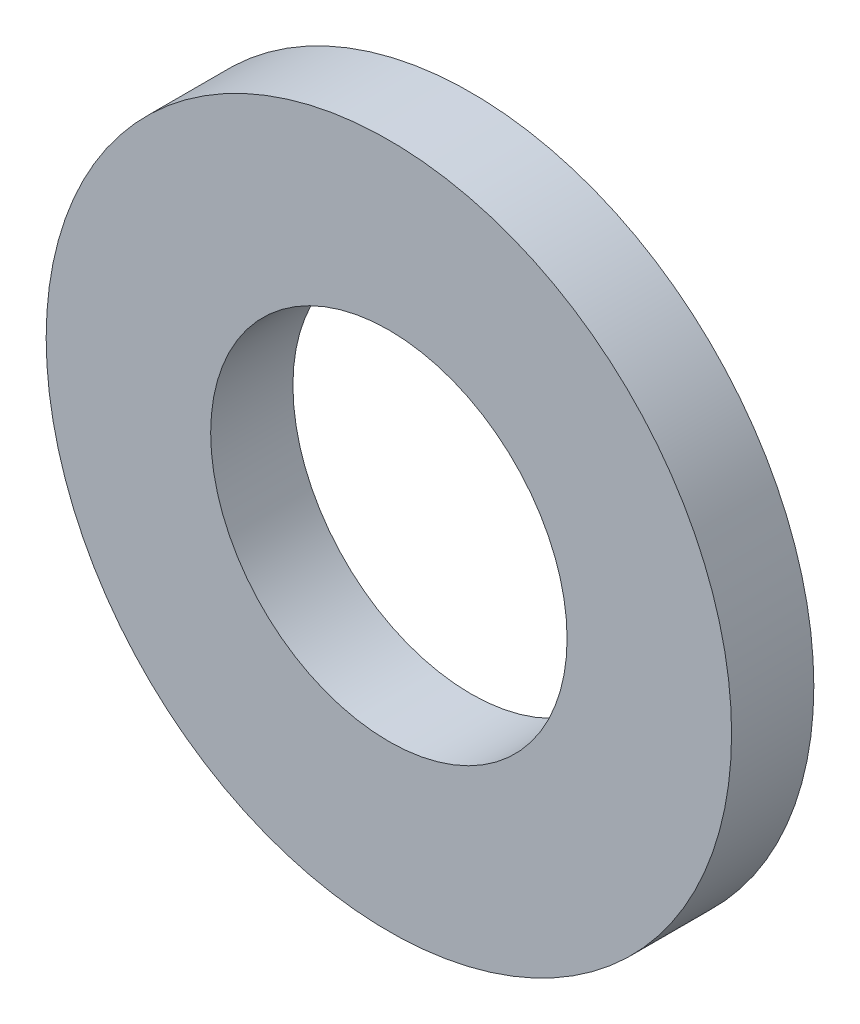
from build123d import *

# Parameters (mm, degrees)
SKETCH1_R           = 12.5
SKETCH1_R_2         = 6.5
BOSS_EXTRUDE1_DEPTH = 3


with BuildPart() as part:
    # Sketch1 → Boss-Extrude1 (new body)
    with BuildSketch(Plane.XY):
        Circle(SKETCH1_R)
        Circle(SKETCH1_R_2, mode=Mode.SUBTRACT)
    extrude(amount=BOSS_EXTRUDE1_DEPTH)


solid = part.part
